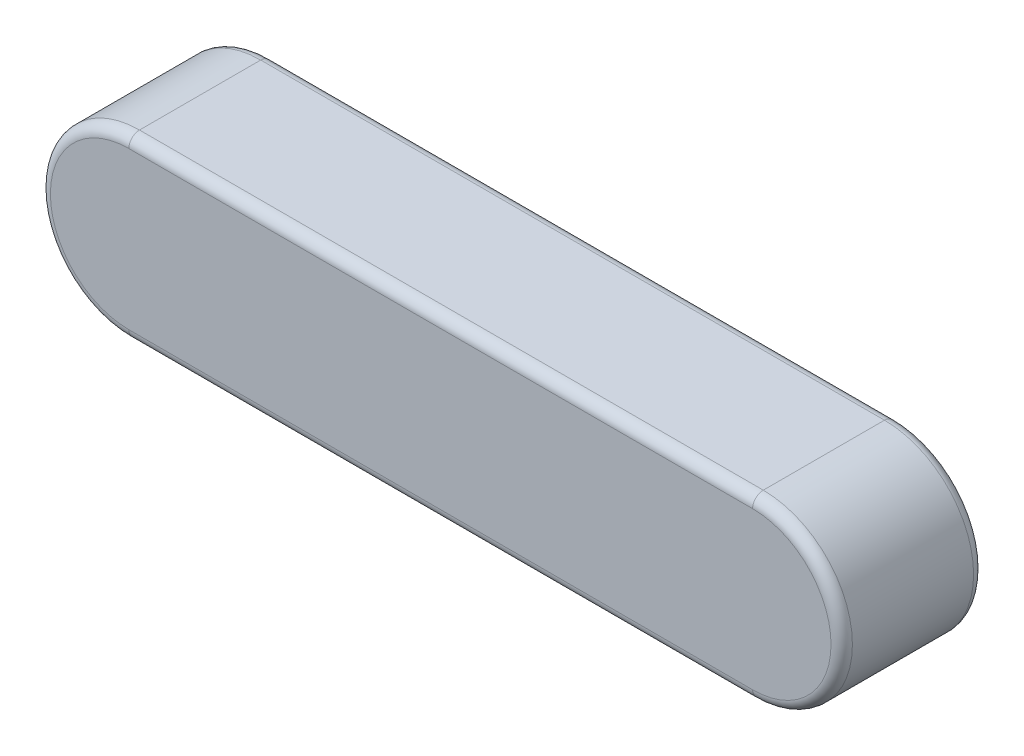
SolidWorks part; units mm, degrees
material "45"
ref_plane "基准面1" through (0, 0, 0) normal (0, 0, 1) x (1, 0, 0)
ref_plane "基准面2" through (0, 0, 0) normal (0, 1, 0) x (1, 0, 0)
ref_plane "基准面3" through (0, 0, 0) normal (1, 0, 0) x (0, 0, -1)
sketch "尺寸草图" plane through (0, 0, 0) normal (0, 0, 1) x (1, 0, 0)
  line L0 (-28, 0) -> (28, 0) construction
  point P3 (-8, 0)
  point P4 (-0.6, 0)
  point P5 (0, 0)
  point P8 (-10, 0)
  point P11 (0, 0)
sketch "草图1" plane through (0, 0, 0) normal (0, 0, 1) x (1, 0, 0)
  line L0 (-28.0599, 0) -> (30.562, 0) construction
  line L1 (-17.5, 5) -> (17.5, 5)
  line L2 (-17.5, -5) -> (17.5, -5)
  line L3 (0, 2.9108) -> (0, -2.1805) construction
  arc A0 (-17.5, 5) -> (-17.5, -5) centre (-17.5, 0) ccw
  arc A1 (17.5, 5) -> (17.5, -5) centre (17.5, 0) cw
extrude "基体-拉伸" add sketch "草图1" along normal blind 8
fillet "圆角1" radius 0.6 8 edges at (22.5, 0, 8) (0, 5, 8) (-22.5, 0, 8) (0, 5, 0) (22.5, 0, 0) (0, -5, 0) (-22.5, 0, 0) (0, -5, 8)
equation "\"D1@草图1\" = \"b@尺寸草图\" / 2"
equation "\"D1@圆角1\" = \"r@尺寸草图\""
equation "\"D1@基体-拉伸\" = \"h@尺寸草图\""
